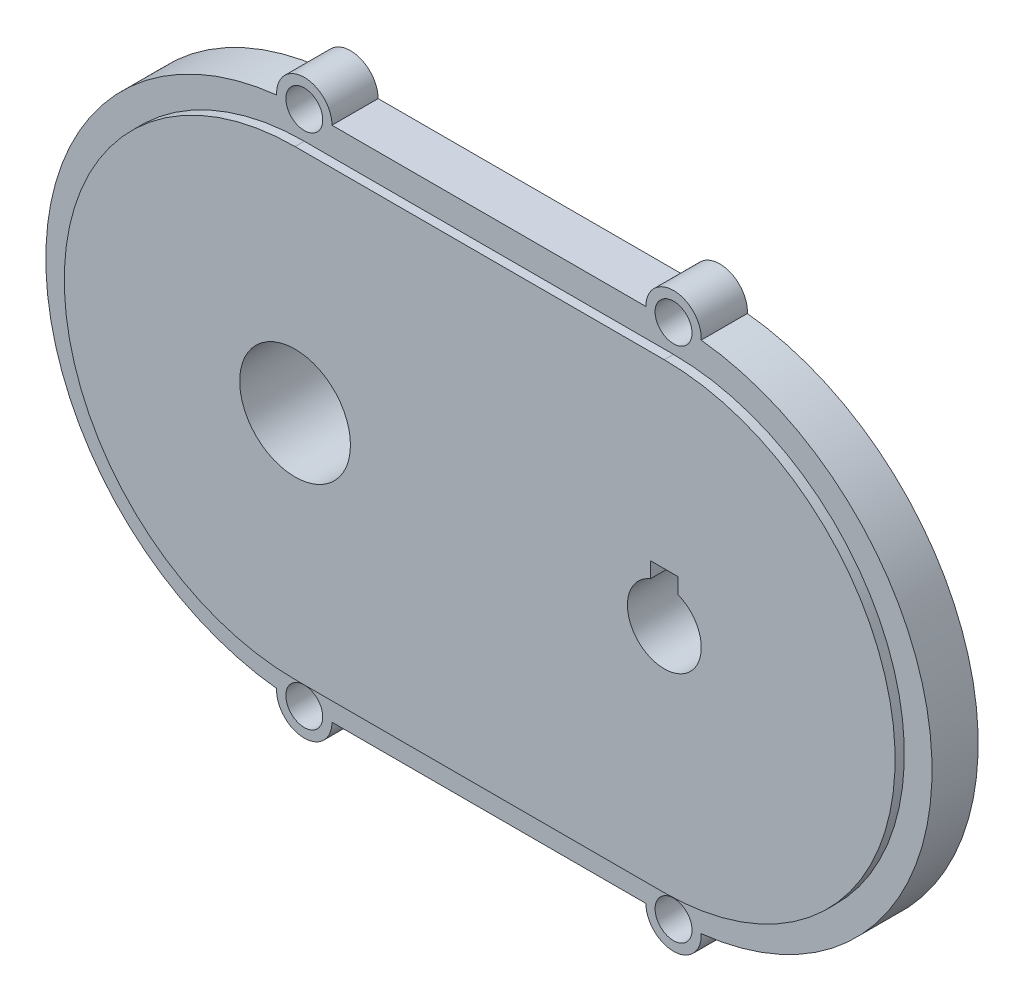
SolidWorks part; units mm, degrees
ref_plane "Front Plane" through (0, 0, 0) normal (0, 0, 1) x (1, 0, 0)
ref_plane "Top Plane" through (0, 0, 0) normal (0, 1, 0) x (1, 0, 0)
ref_plane "Right Plane" through (0, 0, 0) normal (1, 0, 0) x (0, 0, -1)
other "Configuration Table"
sketch "Sketch2" plane through (0, 0, 0) normal (0, 0, 1) x (1, 0, 0)
  line L0 (0, -25.8937) -> (0, 25.8937) construction
  line L1 (-20, 0) -> (20, 0) construction
  line L2 (-20, 28) -> (20, 28)
  line L3 (-20, -28) -> (20, -28)
  arc A0 (-20, 28) -> (-20, -28) centre (-20, 0) ccw
  arc A1 (20, -28) -> (20, 28) centre (20, 0) ccw
  point P4 (0, 0)
  point P7 (0, 0)
  dimension "D2" = 28
  dimension "D1" = 40
extrude "Boss-Extrude1" add sketch "Sketch2" along normal blind 5
sketch "Sketch4" plane through (0, 0, 5) normal (0, 0, 1) x (1, 0, 0)
  line L0 (0, -33.1038) -> (0, 33.1038) construction
  line L1 (-20, 0) -> (20, 0) construction
  line L2 (-20, 25) -> (20, 25)
  line L3 (-20, -25) -> (20, -25)
  arc A0 (-20, 25) -> (-20, -25) centre (-20, 0) ccw
  arc A1 (20, -25) -> (20, 25) centre (20, 0) ccw
  point P4 (0, 0)
  point P7 (0, 0)
  dimension "D2" = 25
  dimension "D1" = 40
extrude "Boss-Extrude2" add sketch "Sketch4" along normal blind 1
sketch "Sketch5" plane through (0, 0, 0) normal (0, 0, -1) x (-1, 0, 0)
  circle A0 centre (-20, 28) radius 3
  circle A1 centre (20, 28) radius 3
  circle A2 centre (-20, -28) radius 3
  circle A3 centre (20, -28) radius 3
  dimension "D1" = 6
  dimension "D2" = 6
extrude "Boss-Extrude3" add sketch "Sketch5" against normal blind 5
sketch "Sketch6" plane through (0, 0, 0) normal (0, 0, -1) x (-1, 0, 0)
  circle A0 centre (-20, 28) radius 2
  circle A1 centre (20, 28) radius 2
  circle A2 centre (-20, -28) radius 2
  circle A3 centre (20, -28) radius 2
  dimension "D1" = 4
extrude "Cut-Extrude1" cut sketch "Sketch6" against normal blind 5
sketch "Sketch7" plane through (0, 0, 0) normal (0, 0, -1) x (-1, 0, 0)
  circle A0 centre (-20, 0) radius 6
  circle A1 centre (20, 0) radius 8
  dimension "D1" = 12
  dimension "D2" = 16
extrude "Boss-Extrude4" add sketch "Sketch7" along normal blind 8
sketch "Sketch8" plane through (0, 0, 6) normal (0, 0, 1) x (1, 0, 0)
  circle A0 centre (-20, 0) radius 6
  circle A1 centre (20, 0) radius 4
  dimension "D1" = 8
  dimension "D2" = 12
extrude "Cut-Extrude2" cut sketch "Sketch8" against normal blind 11
ref_plane "Plane1" through (0, 4, 0) normal (0, 1, 0) x (1, 0, 0)
sketch "Sketch9" plane through (0, 4, 0) normal (0, 1, 0) x (1, 0, 0)
  line L0 (20, -6) -> (20, -5) construction
  line L1 (20, -11.7016) -> (20, 13.8404) construction
  line L2 (16, 5) -> (24, 5) construction
  line L3 (16, 5) -> (24, 5) construction
  line L4 (20, -7.9701) -> (20, 1.6) construction
  line L5 (18.5, -7.9701) -> (18.5, 1.6)
  line L6 (21.5, -7.9701) -> (21.5, 1.6)
  arc A0 (18.5, -7.9701) -> (21.5, -7.9701) centre (20, -7.9701) ccw
  arc A1 (21.5, 1.6) -> (18.5, 1.6) centre (20, 1.6) ccw
  point P2 (20, -3.185)
  dimension "D1" = 1.5
  dimension "D2" = 3.4
extrude "Cut-Extrude3" cut sketch "Sketch9" against normal mid plane 2.8
